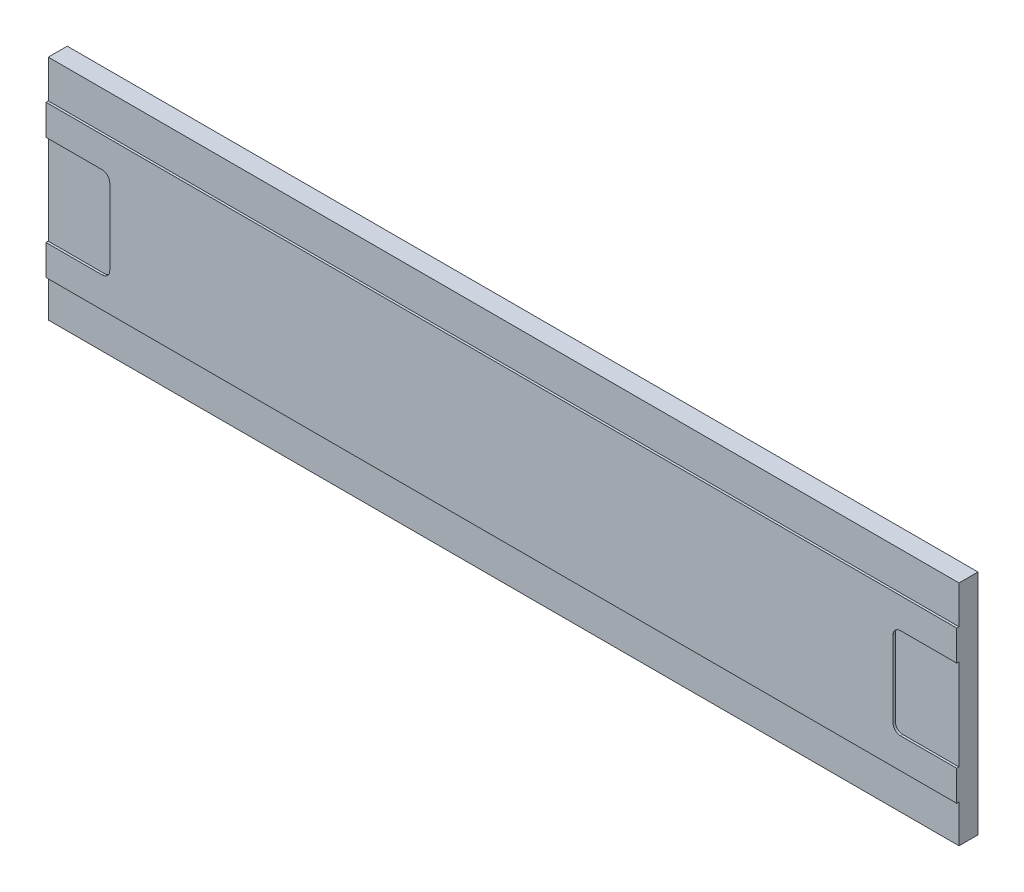
from build123d import *

# Parameters (mm, degrees)
SKETCH_1_W          = 600
SKETCH_1_H          = 150
EXTRUDE_1_DEPTH     = 14
SKETCH_2_W          = 600
SKETCH_2_H          = 25
CUT_EXTRUDE_1_DEPTH = 1.5
SKETCH_3_W          = 42
SKETCH_3_H          = 60
CUT_EXTRUDE_2_DEPTH = 1.5
FILLET_1_R          = 5


with BuildPart() as part:
    # 草图1 → 凸台-拉伸1 (new body)
    with BuildSketch(Plane.XY):
        Rectangle(SKETCH_1_W, SKETCH_1_H)
    extrude(amount=EXTRUDE_1_DEPTH)

    # 草图2 → 切除-拉伸1 (cut)
    with BuildSketch(Plane.XY.offset(14)):
        with Locations((0, 62.5)):
            Rectangle(SKETCH_2_W, SKETCH_2_H)
        with Locations((0, -62.5)):
            Rectangle(SKETCH_2_W, SKETCH_2_H)
    extrude(amount=-CUT_EXTRUDE_1_DEPTH, mode=Mode.SUBTRACT)

    # 草图3 → 切除-拉伸2 (cut)
    with BuildSketch(Plane.XY.offset(14)):
        with Locations((-279, 0)):
            Rectangle(SKETCH_3_W, SKETCH_3_H)
        with Locations((279, 0)):
            Rectangle(SKETCH_3_W, SKETCH_3_H)
    extrude(amount=-CUT_EXTRUDE_2_DEPTH, mode=Mode.SUBTRACT)

    # 圆角1
    fillet_1_edges = [part.edges().sort_by_distance(p)[0] for p in [
        (-258, 30, 13.25),
        (-258, -30, 13.25),
        (258, -30, 13.25),
        (258, 30, 13.25),
    ]]
    fillet(fillet_1_edges, radius=FILLET_1_R)


solid = part.part
